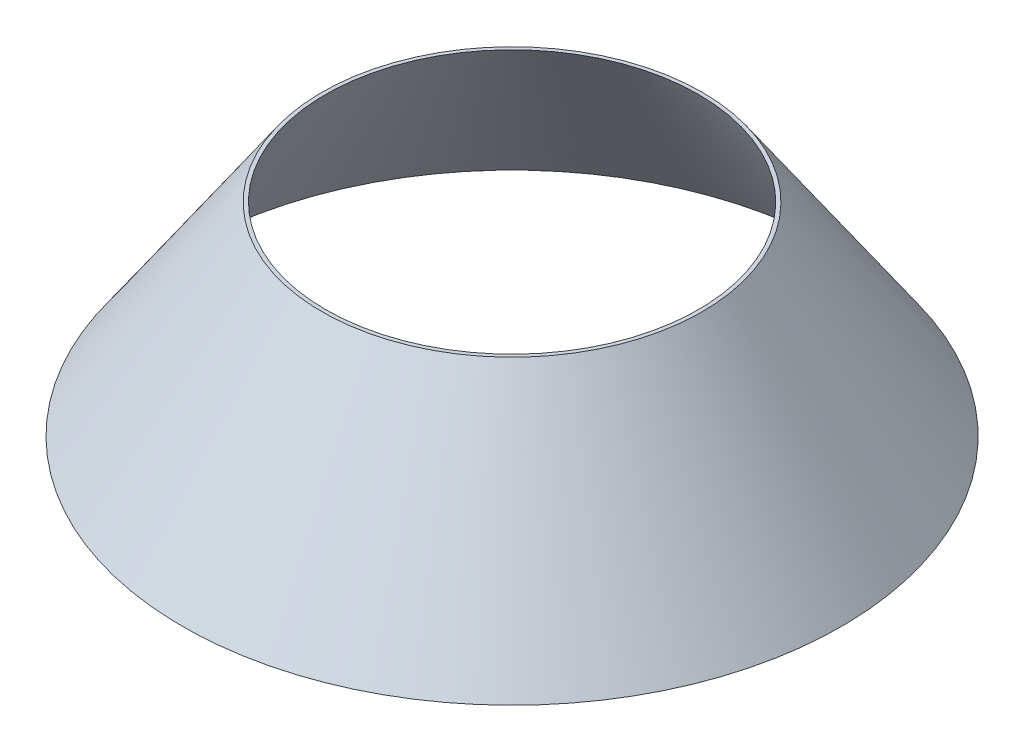
from build123d import *

# Parameters (mm, degrees)
SHELL1_T = -1.2


with BuildPart() as part:
    # Sketch3 → Revolve1 (revolve)
    with BuildSketch(Plane.XY, mode=Mode.PRIVATE) as revolve1_sk:
        Polygon((0, 80), (75, 80), (130, 0), (0, 0), align=None)
    revolve(revolve1_sk.sketch.rotate(Axis((0, 0, 0), (0, 1, 0)), 90), axis=Axis((0, 0, 0), (0, 1, 0)))

    # Shell1
    shell1_openings = [part.faces().sort_by_distance(p)[0] for p in [
        (0, 0, 0),
        (0, 80, 0),
    ]]
    offset(amount=SHELL1_T, openings=shell1_openings, kind=Kind.INTERSECTION)


solid = part.part
